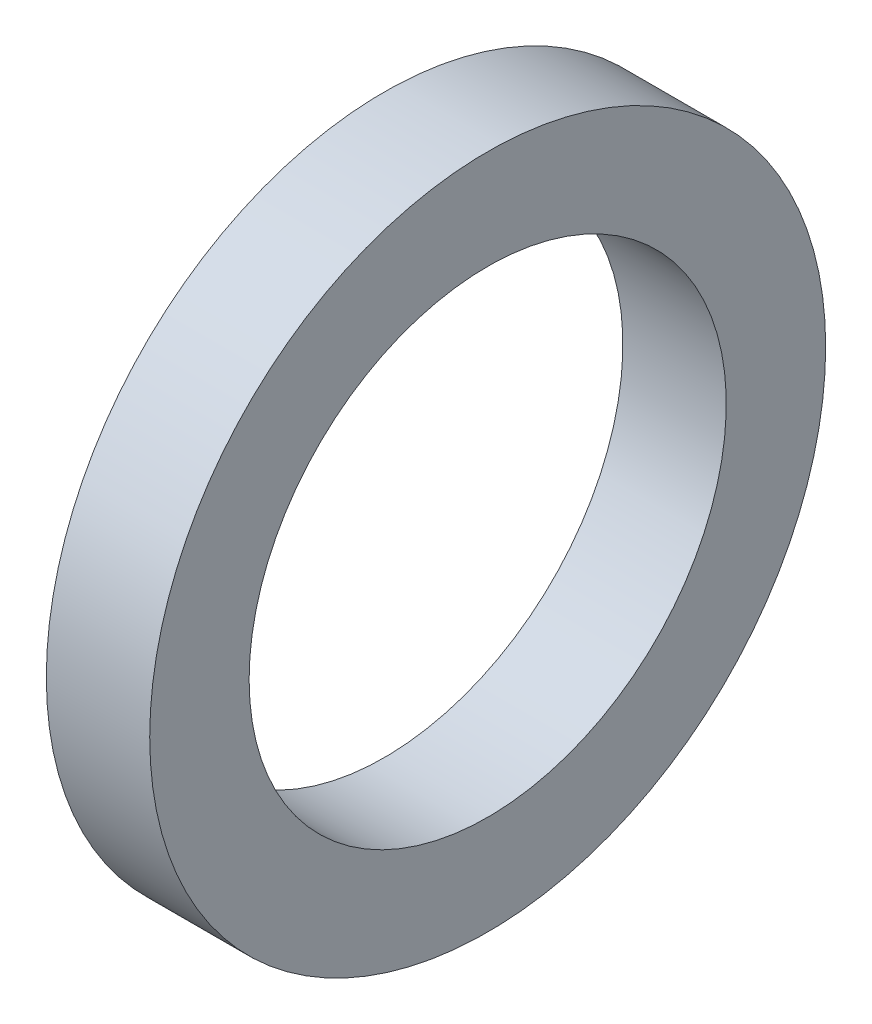
from build123d import *

# Parameters (mm, degrees)
SKETCH_1_R      = 42.5
SKETCH_1_R_2    = 30
EXTRUDE_1_DEPTH = 13


with BuildPart() as part:
    # 草图1 → 凸台-拉伸1 (new body)
    with BuildSketch(Plane(origin=(0, 0, 0), x_dir=(0, 0, -1), z_dir=(1, 0, 0))):
        with Locations(Location((0, 0, 0), (0, 0, 180))):
            Circle(SKETCH_1_R)
        with Locations(Location((0, 0, 0), (0, 0, 180))):
            Circle(SKETCH_1_R_2, mode=Mode.SUBTRACT)
    extrude(amount=EXTRUDE_1_DEPTH)


solid = part.part
